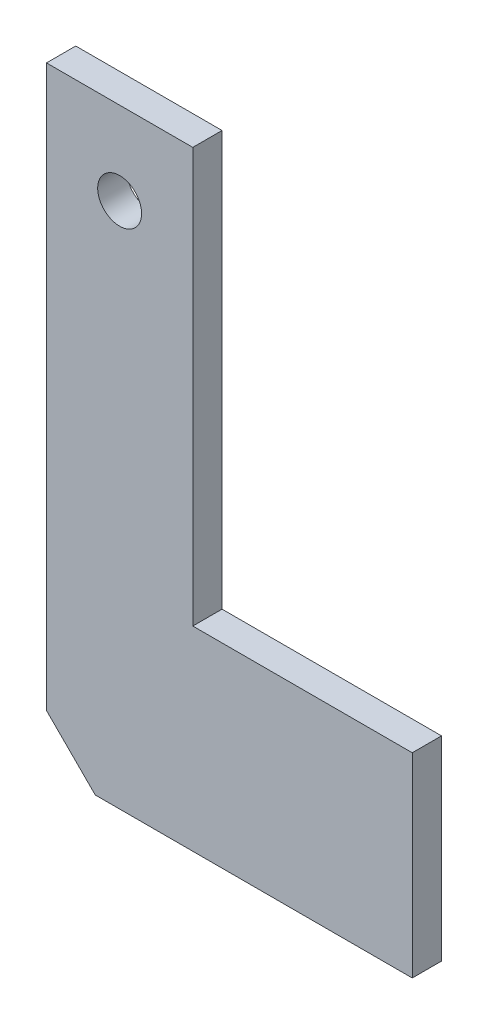
from build123d import *

# Parameters (mm, degrees)
BOSS_EXTRUDE1_DEPTH = 6
CUT_EXTRUDE1_REACH  = 98.228
SKETCH2_R           = 4.5
CHAMFER1_SIZE       = 10


with BuildPart() as part:
    # Sketch1 → Boss-Extrude1 (new body)
    with BuildSketch(Plane.XY):
        Polygon((-33.521587555, -86.6224812), (-33.521587555, 38.3775188), (-3.521587555, 38.3775188), (-3.521587555, -46.6224812), (41.478412445, -46.6224812), (41.478412445, -86.6224812), align=None)
    extrude(amount=BOSS_EXTRUDE1_DEPTH)

    # Sketch2 → Cut-Extrude1 (cut, up to next)
    with BuildSketch(Plane.XY.offset(6), mode=Mode.PRIVATE) as cut_extrude1_sk1:
        with Locations((-18.521587555, 21.3775188)):
            Circle(SKETCH2_R)
    cut_extrude1_tool1 = extrude(cut_extrude1_sk1.sketch, amount=-CUT_EXTRUDE1_REACH, mode=Mode.PRIVATE) & part.part
    add(cut_extrude1_tool1.solids().sort_by_distance((-18.521588, 21.377519, 6))[0], mode=Mode.SUBTRACT)

    # Chamfer1
    chamfer1_edges = [part.edges().sort_by_distance(p)[0] for p in [
        (-33.521587555, -86.6224812, 3),
    ]]
    chamfer(chamfer1_edges, length=CHAMFER1_SIZE)


solid = part.part
